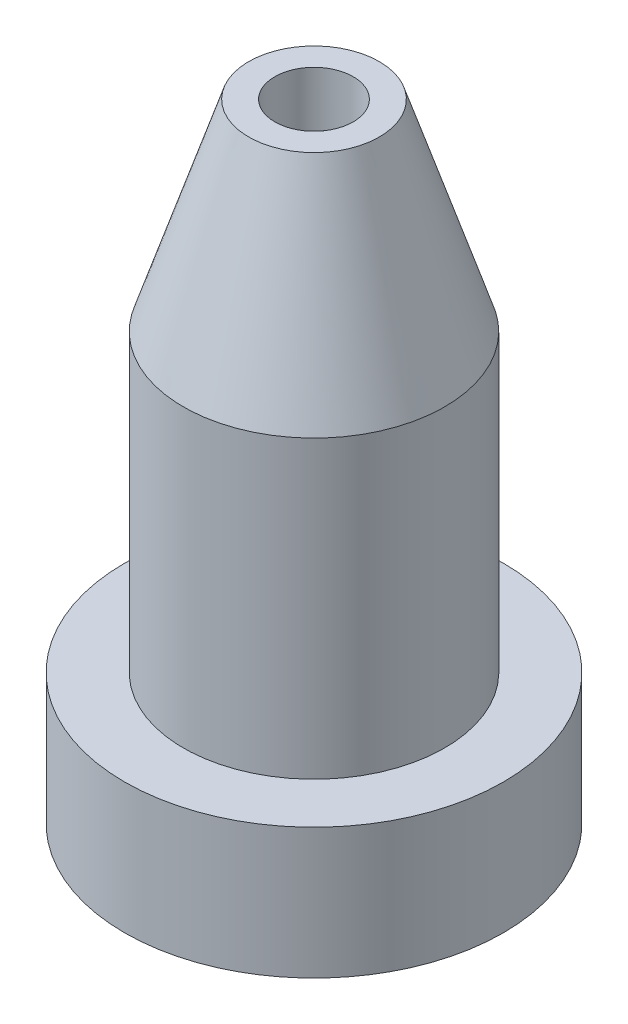
SolidWorks part; units mm, degrees
ref_plane "Front Plane" through (0, 0, 0) normal (0, 0, 1) x (1, 0, 0)
ref_plane "Top Plane" through (0, 0, 0) normal (0, 1, 0) x (1, 0, 0)
ref_plane "Right Plane" through (0, 0, 0) normal (1, 0, 0) x (0, 0, -1)
sketch "Sketch1" plane through (0, 0, 0) normal (0, 1, 0) x (1, 0, 0)
  circle A0 centre (0, 0) radius 1
  dimension "D1" = 2
extrude "Boss-Extrude1" add sketch "Sketch1" along normal blind 4.8
sketch "Sketch2" plane through (0, 0, 0) normal (0, 0, 1) x (1, 0, 0)
  line L0 (0, 0) -> (0, 50000) construction
  line L1 (0.5, 4.8) -> (1.6214, 1.3486)
  line L2 (1, 4.8) -> (-1, 4.8) construction
  line L4 (0.5, 4.8) -> (1.6214, 4.8)
  line L5 (1.6214, 4.8) -> (1.6214, 1.3486)
  dimension "D1" = 1
  dimension "D2" = 18
revolve "Cut-Revolve1" cut sketch "Sketch2" angle 360 about L0
sketch "Sketch3" plane through (0, 0, 0) normal (0, -1, 0) x (1, 0, 0)
  circle A0 centre (0, 0) radius 0.75
  dimension "D1" = 1.5
extrude "Cut-Extrude1" cut sketch "Sketch3" against normal blind 3
sketch "Sketch4" plane through (0, 4.8, 0) normal (0, 1, 0) x (1, 0, 0)
  circle A0 centre (0, 0) radius 0.3
  dimension "D1" = 0.6
extrude "Cut-Extrude2" cut sketch "Sketch4" against normal blind 3
sketch "Sketch5" plane through (0, 3, 0) normal (0, -1, 0) x (1, 0, 0)
  circle A0 centre (0, 0) radius 0.5
  dimension "D1" = 1
extrude "Cut-Extrude3" cut sketch "Sketch5" against normal blind 0.6
sketch "Sketch6" plane through (0, 0, 0) normal (0, -1, 0) x (1, 0, 0)
  circle A0 centre (0, 0) radius 1.45
  circle A1 centre (0, 0) radius 1 construction
  circle A2 centre (0, 0) radius 1
  dimension "D1" = 2.9
extrude "Boss-Extrude2" add sketch "Sketch6" against normal blind 1
chamfer "Chamfer1" distance 0.3 distance2 1 1 edges at (0, 0, -0.75)
